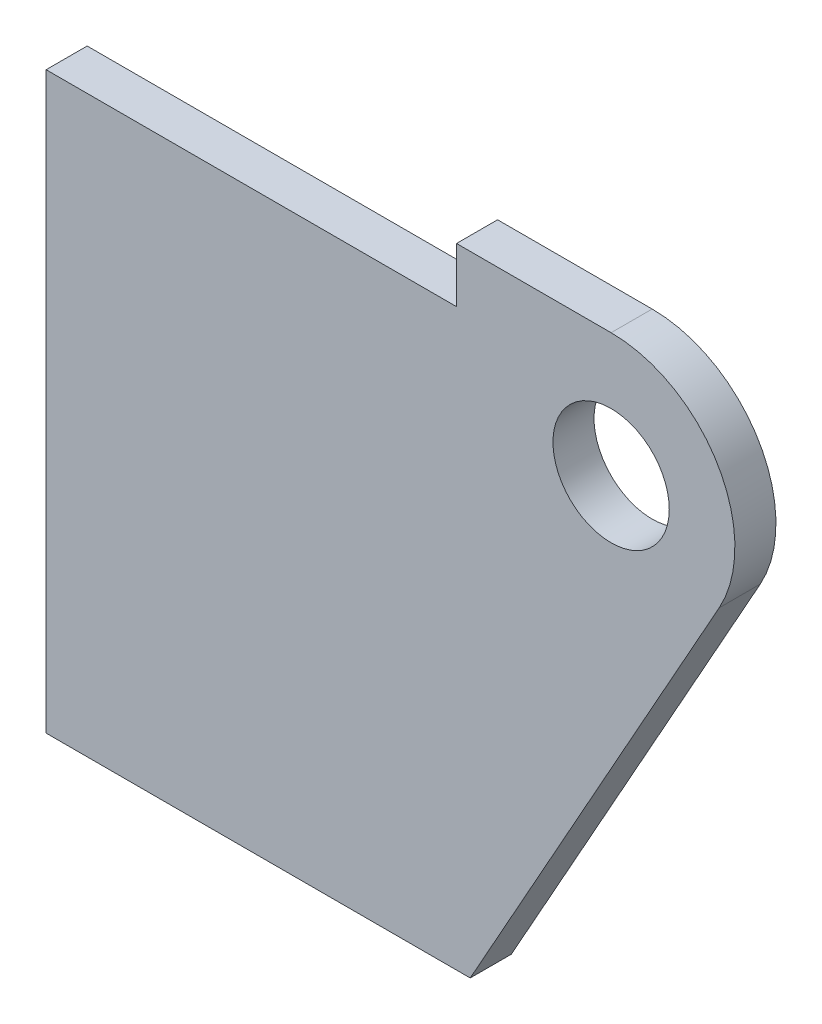
from build123d import *

# Parameters (mm, degrees)
SKETCH1_R           = 42.5
BOSS_EXTRUDE1_DEPTH = 30


with BuildPart() as part:
    # Sketch1 → Boss-Extrude1 (new body)
    with BuildSketch(Plane.XY):
        with BuildLine():
            Line((0, 0), (0, 420))
            Line((0, 420), (300, 420))
            Line((300, 420), (300, 460))
            Line((300, 460), (413, 460))
            ThreePointArc((413, 460), (491.066504669, 415.280682048), (491.982051466, 325.317587819))
            Line((491.982051466, 325.317587819), (310, 0))
            Line((310, 0), (0, 0))
        make_face()
        with Locations((413, 369.5)):
            Circle(SKETCH1_R, mode=Mode.SUBTRACT)
    extrude(amount=BOSS_EXTRUDE1_DEPTH)


solid = part.part
